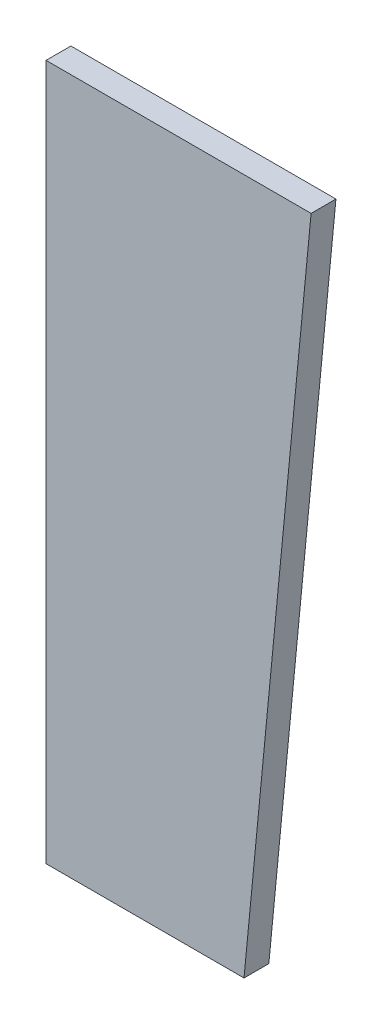
from build123d import *

# Parameters (mm, degrees)
BOSS_EXTRUDE1_DEPTH = 30


with BuildPart() as part:
    # Sketch1 → Boss-Extrude1 (new body)
    with BuildSketch(Plane.XY):
        Polygon((0, 0), (239, 0), (320, 840), (0, 840), align=None)
    extrude(amount=BOSS_EXTRUDE1_DEPTH)


solid = part.part
